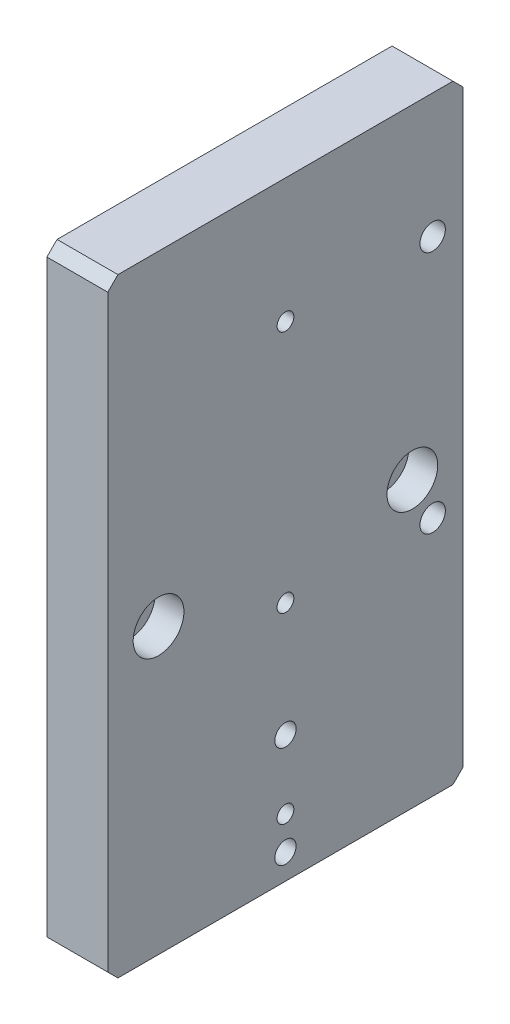
from build123d import *

# Parameters (mm, degrees)
SKETCH1_W                                            = 70
SKETCH1_H                                            = 120
BOSS_EXTRUDE1_DEPTH                                  = 12
M5_TAPPED_HOLE1_D                                    = 4.2
M5_TAPPED_HOLE1_DEPTH                                = 12.4
M5_TAPPED_HOLE1_TIP                                  = 1.2618073
CBORE_FOR_M5_HEXAGON_SOCKET_HEAD_CAP_SCR_D           = 5.5
CBORE_FOR_M5_HEXAGON_SOCKET_HEAD_CAP_SCR_CBORE_D     = 10
CBORE_FOR_M5_HEXAGON_SOCKET_HEAD_CAP_SCR_CBORE_DEPTH = 5.7
M4_TAPPED_HOLE1_D                                    = 3.3
M4_TAPPED_HOLE1_DEPTH                                = 10.1
M4_TAPPED_HOLE1_TIP                                  = 0.991420021
F_5_0MM_DOWEL_HOLE1_D                                = 5
F_5_0MM_DOWEL_HOLE1_DEPTH                            = 8
F_5_0MM_DOWEL_HOLE1_TIP                              = 1.502151548
CHAMFER1_SIZE                                        = 2


with BuildPart() as part:
    # Sketch1 → Boss-Extrude1 (new body)
    with BuildSketch(Plane(origin=(0, 0, 0), x_dir=(0, 0, -1), z_dir=(1, 0, 0))):
        Rectangle(SKETCH1_W, SKETCH1_H)
    extrude(amount=BOSS_EXTRUDE1_DEPTH)

    # M5 Tapped Hole1
    with Locations(Plane.ZY):
        with Locations((0, -35), (0, -55)):
            Hole(M5_TAPPED_HOLE1_D / 2, depth=M5_TAPPED_HOLE1_DEPTH)
            with Locations((0, 0, -(M5_TAPPED_HOLE1_DEPTH + M5_TAPPED_HOLE1_TIP / 2))):  # 118° drill point
                Cone(0, M5_TAPPED_HOLE1_D / 2, M5_TAPPED_HOLE1_TIP, mode=Mode.SUBTRACT)

    # CBORE for M5 Hexagon socket head cap screws1 (through all)
    with Locations(Plane(origin=(12, 0, 0), x_dir=(0, 0, -1), z_dir=(1, 0, 0))):
        with Locations((25, -4), (-25, -4)):
            CounterBoreHole(CBORE_FOR_M5_HEXAGON_SOCKET_HEAD_CAP_SCR_D / 2, CBORE_FOR_M5_HEXAGON_SOCKET_HEAD_CAP_SCR_CBORE_D / 2, CBORE_FOR_M5_HEXAGON_SOCKET_HEAD_CAP_SCR_CBORE_DEPTH)

    # M4 Tapped Hole1
    with Locations(Plane(origin=(12, 0, 0), x_dir=(0, 0, -1), z_dir=(1, 0, 0))):
        with Locations((0, -48.5), (0, -12.5), (0, 35.5)):
            Hole(M4_TAPPED_HOLE1_D / 2, depth=M4_TAPPED_HOLE1_DEPTH)
            with Locations((0, 0, -(M4_TAPPED_HOLE1_DEPTH + M4_TAPPED_HOLE1_TIP / 2))):  # 118° drill point
                Cone(0, M4_TAPPED_HOLE1_D / 2, M4_TAPPED_HOLE1_TIP, mode=Mode.SUBTRACT)

    # Ø5.0mm Dowel Hole1
    with Locations(Plane(origin=(12, 0, 0), x_dir=(0, 0, -1), z_dir=(1, 0, 0))):
        with Locations((29, 35.5), (29, -12.5)):
            Hole(F_5_0MM_DOWEL_HOLE1_D / 2, depth=F_5_0MM_DOWEL_HOLE1_DEPTH)
            with Locations((0, 0, -(F_5_0MM_DOWEL_HOLE1_DEPTH + F_5_0MM_DOWEL_HOLE1_TIP / 2))):  # 118° drill point
                Cone(0, F_5_0MM_DOWEL_HOLE1_D / 2, F_5_0MM_DOWEL_HOLE1_TIP, mode=Mode.SUBTRACT)

    # Chamfer1
    chamfer1_edges = [part.edges().sort_by_distance(p)[0] for p in [
        (6, -60, -35),
        (6, -60, 35),
        (6, 60, 35),
        (6, 60, -35),
    ]]
    chamfer(chamfer1_edges, length=CHAMFER1_SIZE)


solid = part.part
